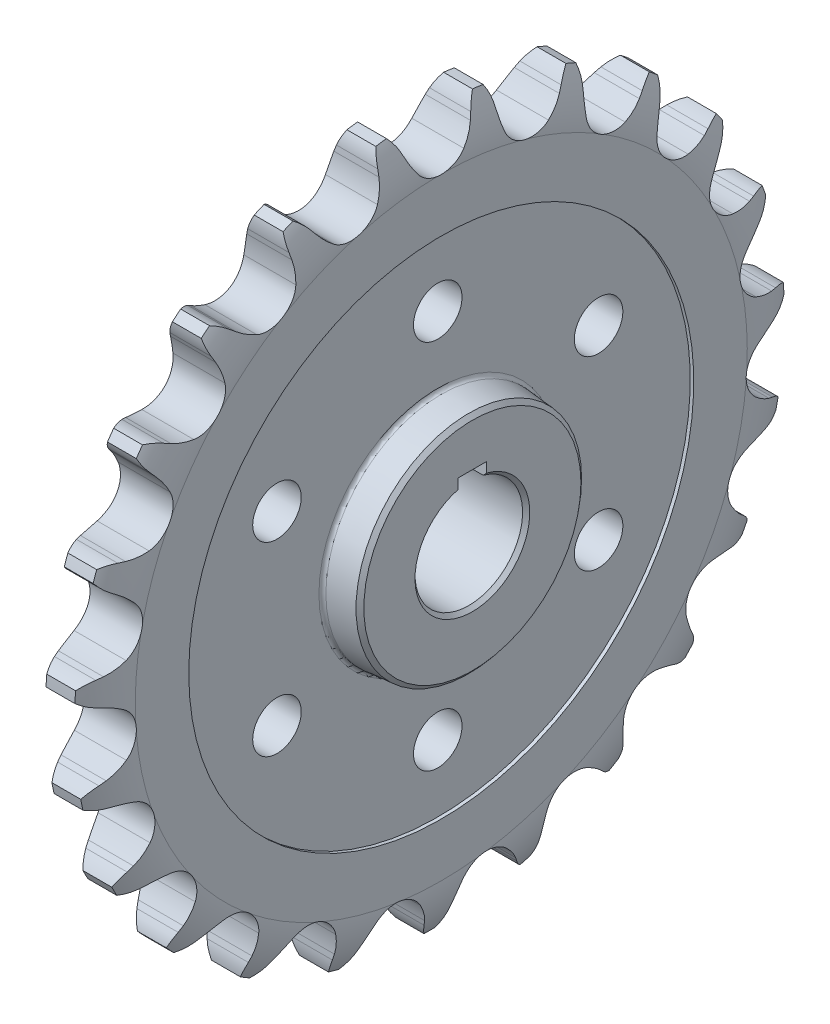
from build123d import *
from OCP.BRepFilletAPI import BRepFilletAPI_MakeChamfer

# Parameters (mm, degrees)
CUT_EXTRUDE_1_DEPTH      = 10.985625
PATTERN_CIRCULAR_1_COUNT = 23
SKETCH_4_W               = 8
SKETCH_4_H               = 3.843167657
CUT_EXTRUDE_2_DEPTH      = 142.682304467
FILLET_1_R               = 1.016
CHAMFER_1_SIZE           = 1
CHAMFER_1_SIZE2          = 1.100062868
SKETCH_6_R               = 6.766276752
CUT_EXTRUDE_3_DEPTH      = 142.682304467
PATTERN_CIRCULAR_2_COUNT = 6


with BuildPart() as part:
    # 草图1 → 旋转1 (revolve)
    with BuildSketch(Plane.XY, mode=Mode.PRIVATE) as revolve_1_sk:
        with BuildLine():
            Line((-6.35, 15), (-6.35, 70.408065891))
            Line((-6.35, 70.408065891), (-7.32375, 70.408065891))
            Line((-7.32375, 70.408065891), (-7.32375, 85.328065891))
            ThreePointArc((-7.32375, 85.328065891), (-6.637955477, 92.397146158), (-4.02175, 99))
            Line((-4.02175, 99), (4.02175, 99))
            ThreePointArc((4.02175, 99), (6.637955477, 92.397146158), (7.32375, 85.328065891))
            Line((7.32375, 85.328065891), (7.32375, 70.408065891))
            Line((7.32375, 70.408065891), (6.35, 70.408065891))
            Line((6.35, 70.408065891), (6.35, 15))
            Line((6.35, 15), (-6.35, 15))
        make_face()
    revolve(revolve_1_sk.sketch.rotate(Axis((-12.7, 0, 0), (1, 0, 0)), 90), axis=Axis((-12.7, 0, 0), (1, 0, 0)))

    # 草图2 → 切除-拉伸1 (cut, symmetric)
    with BuildSketch(Plane(origin=(0, 0, 0), x_dir=(0, 0, -1), z_dir=(1, 0, 0))):
        with BuildLine():
            Line((9.153981346, 93.239311175), (9.777473277, 94.779142626))
            ThreePointArc((9.777473277, 94.779142626), (10.726859473, 96.625281975), (11.99226046, 98.27098091))
            ThreePointArc((11.99226046, 98.27098091), (0, 99), (-11.99226046, 98.27098091))
            ThreePointArc((-11.99226046, 98.27098091), (-10.726859473, 96.625281975), (-9.777473277, 94.779142626))
            Line((-9.777473277, 94.779142626), (-9.153981346, 93.239311175))
            ThreePointArc((-9.153981346, 93.239311175), (-7.923224103, 90.708577785), (-6.361104523, 88.367817801))
            ThreePointArc((-6.361104523, 88.367817801), (0, 85.238365891), (6.361104523, 88.367817801))
            ThreePointArc((6.361104523, 88.367817801), (7.923224103, 90.708577785), (9.153981346, 93.239311175))
        make_face()
    cut_extrude_1 = extrude(amount=CUT_EXTRUDE_1_DEPTH, both=True, mode=Mode.SUBTRACT)

    # 阵列(圆周)1: 切除-拉伸1 ×23 about axis
    pattern_circular_1_axis = Axis((0, 0, 0), (1, 0, 0))
    for i in range(1, PATTERN_CIRCULAR_1_COUNT):
        add(cut_extrude_1.rotate(pattern_circular_1_axis, i * 360 / PATTERN_CIRCULAR_1_COUNT), mode=Mode.SUBTRACT)

    # 草图5 → 旋转2 (revolve)
    with BuildSketch(Plane.XY, mode=Mode.PRIVATE) as revolve_2_sk:
        Polygon((-16, 15), (16, 15), (16, 31.365361318), (6.35, 32.209626921), (-6.35, 32.209626921), (-16, 31.365361318), align=None)
    revolve(revolve_2_sk.sketch.rotate(Axis((0, 0, 0), (-1, 0, 0)), 90), axis=Axis((0, 0, 0), (-1, 0, 0)))

    # 草图4 → 切除-拉伸2 (cut, through all)
    with BuildSketch(Plane.ZY.offset(6.35)):
        with Locations((0, 16.378416124)):
            Rectangle(SKETCH_4_W, SKETCH_4_H)
    cut_extrude_2 = extrude(amount=-CUT_EXTRUDE_2_DEPTH, mode=Mode.SUBTRACT)

    # 镜向1: 切除-拉伸2 across plane
    add(cut_extrude_2.mirror(Plane(origin=(0, 0, 0), x_dir=(0, 0, 1), z_dir=(1, 0, 0))), mode=Mode.SUBTRACT)

    # 圆角1
    fillet_1_edges = [part.edges().sort_by_distance(p)[0] for p in [
        (-6.35, 0, 32.209626921),
        (6.35, 0, 32.209626921),
    ]]
    fillet(fillet_1_edges, radius=FILLET_1_R)

    # 倒角1: one chamfer whose edges measure the first distance from different faces: ONE call of the kernel's chamfer builder (chamfer() names one face for all edges)
    chamfer_1_edges_1 = [part.edges().sort_by_distance(p)[0] for p in [
        (-16, 0, 31.365361318),
    ]]
    chamfer_1_side_1 = [part.faces().sort_by_distance(p)[0] for p in [
        (-16, 0, 30.478214931),
    ]]
    chamfer_1_edges_2 = [part.edges().sort_by_distance(p)[0] for p in [
        (16, 0, 31.365361318),
    ]]
    chamfer_1_side_2 = [part.faces().sort_by_distance(p)[0] for p in [
        (11.638724883, 0, 31.746923449),
    ]]
    chamfer_1_edges_3 = [part.edges().sort_by_distance(p)[0] for p in [
        (16, -15, 0),
        (-16, -15, 0),
    ]]
    chamfer_1 = BRepFilletAPI_MakeChamfer(part.part.solid().wrapped)
    for e in chamfer_1_edges_1:
        chamfer_1.Add(CHAMFER_1_SIZE, CHAMFER_1_SIZE2, e.wrapped, chamfer_1_side_1[0].wrapped)  # the first distance lies on this face
    for e in chamfer_1_edges_2:
        chamfer_1.Add(CHAMFER_1_SIZE, CHAMFER_1_SIZE2, e.wrapped, chamfer_1_side_2[0].wrapped)  # the first distance lies on this face
    for e in chamfer_1_edges_3:
        chamfer_1.Add(CHAMFER_1_SIZE, e.wrapped)
    add(Compound.cast(chamfer_1.Shape()), mode=Mode.REPLACE)

    # 草图6 → 切除-拉伸3 (cut, through all)
    with BuildSketch(Plane.ZY.offset(6.35)):
        with Locations((0, 51.774342642)):
            Circle(SKETCH_6_R)
    cut_extrude_3 = extrude(amount=-CUT_EXTRUDE_3_DEPTH, mode=Mode.SUBTRACT)

    # 阵列(圆周)2: 切除-拉伸3 ×6 about axis
    pattern_circular_2_axis = Axis((0, 0, 0), (1, 0, 0))
    for i in range(1, PATTERN_CIRCULAR_2_COUNT):
        add(cut_extrude_3.rotate(pattern_circular_2_axis, i * 360 / PATTERN_CIRCULAR_2_COUNT), mode=Mode.SUBTRACT)


solid = part.part
